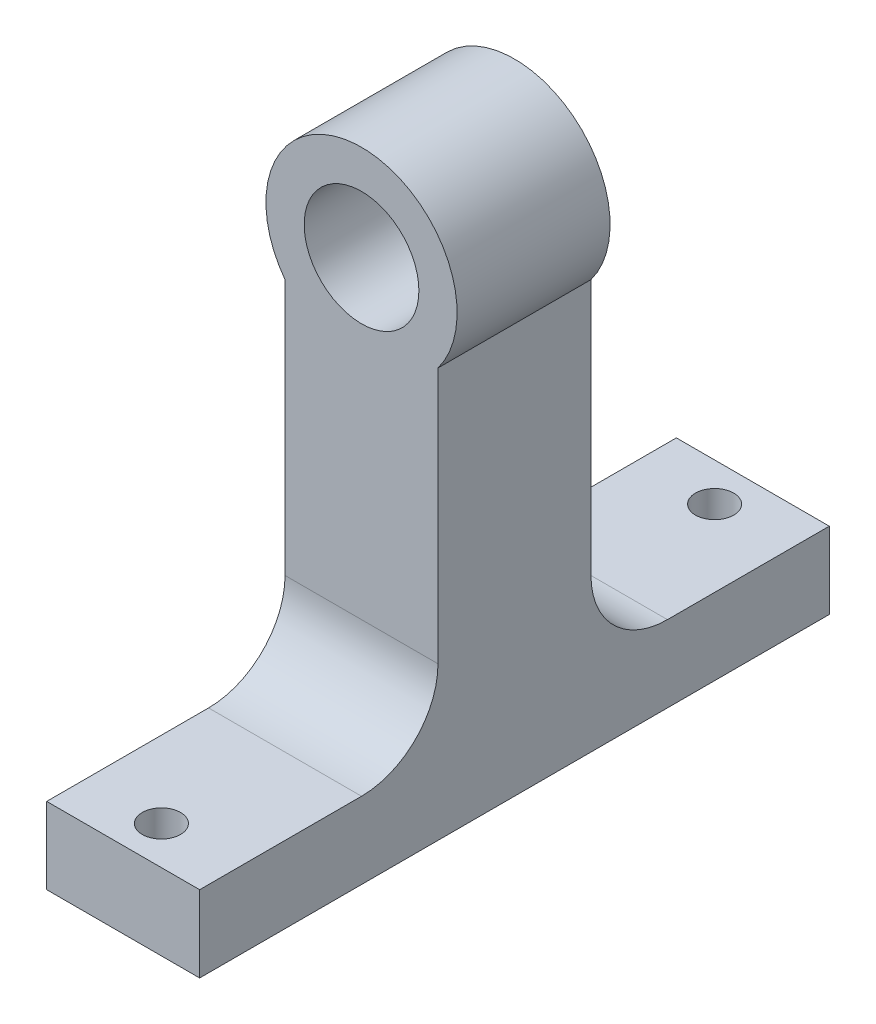
SolidWorks part; units mm, degrees
material "1060 合金"
ref_plane "前视基准面" through (0, 0, 0) normal (0, 0, 1) x (1, 0, 0)
ref_plane "上视基准面" through (0, 0, 0) normal (0, 1, 0) x (1, 0, 0)
ref_plane "右视基准面" through (0, 0, 0) normal (1, 0, 0) x (0, 0, -1)
sketch "草图1" plane through (0, 0, 0) normal (0, 0, 1) x (1, 0, 0)
  circle A0 centre (0, 0) radius 12.5
  circle A1 centre (0, 0) radius 7.5
  dimension "D1" = 15
  dimension "D2" = 25
extrude "凸台-拉伸1" add sketch "草图1" along normal mid plane 20
sketch "草图5" plane through (0, 0, 0) normal (1, 0, 0) x (0, 0, -1)
  line L1 (21.6577, -51) -> (41.1684, -51)
  line L2 (41.1684, -51) -> (41.1684, -61)
  line L3 (41.1684, -61) -> (-41.1684, -61)
  line L5 (10, -12.5) -> (10, -41)
  line L6 (-10, -12.5) -> (10, -12.5)
  line L7 (-41.1684, -51) -> (-41.1684, -61)
  line L8 (-21.6577, -51) -> (-41.1684, -51)
  line L10 (20, -51) -> (21.6577, -51)
  line L11 (-10, -12.5) -> (-10, -41)
  line L12 (-20, -51) -> (-21.6577, -51)
  arc A0 (-20, -51) -> (-10, -41) centre (-20, -41) ccw
  arc A1 (20, -51) -> (10, -41) centre (20, -41) cw
  dimension "D4" = 10
  dimension "D1" = 48.5
  dimension "D2" = 10
  dimension "D3" = 10
extrude "凸台-拉伸3" add sketch "草图5" along normal mid plane 20 separate body
sketch "草图6" plane through (0, -12.5, 0) normal (0, 1, 0) x (1, 0, 0)
  line L4 (-10, 10) -> (-10, -10)
  line L5 (-10, -10) -> (10, -10)
  line L6 (10, -10) -> (10, 10)
  line L7 (-10, -10) -> (10, -10)
  line L8 (-10, 10) -> (-10, -10)
  line L10 (10, -10) -> (10, 10)
  line L12 (10, 10) -> (-10, 10)
  line L13 (10, 10) -> (-10, 10)
  dimension "D1" = 0
extrude "凸台-拉伸4" add sketch "草图6" along normal up to surface up to face at (12.5, 0, 10)
hole_wizard "M6 螺纹孔1" positions "3D草图1" profile "草图8" tap size "M6" standard "GB" end condition up to next
sketch3d "3D草图1"
  line L0 (10, -51, 20) -> (10, -51, 41.1684) construction
  line L1 (10, -51, 41.1684) -> (-10, -51, 41.1684) construction
  point P0 (0, -51, 36.1684)
  dimension "D1" = 10
  dimension "D2" = 5
sketch "草图8" plane through (0, -51, 36.1684) normal (1, 0, 0) x (0, 0, 1)
  line L0 (0, 0) -> (0, 10)
  line L1 (0, 10) -> (2.5, 10)
  line L2 (2.5, 10) -> (2.5, 0)
  line L5 (2.5, 0) -> (0, 0)
  line L11 (0, -6.35) -> (0, 107.95) construction
  dimension "通孔螺纹孔钻头直径" = 5
  dimension "通孔螺纹孔钻头深度" = 10
cosmetic thread "孔螺蚊线1" parameters "D1"=16, "D2"=6
mirror "镜向1" about plane through (0, 0, 0) normal (0, 0, 1) of "M6 螺纹孔1"
sketch "草图9" plane through (0, 0, 10) normal (0, 0, 1) x (1, 0, 0)
  circle A0 centre (0, 0) radius 12.5
  circle A1 centre (0, 0) radius 7.5
  dimension "D1" = 15
